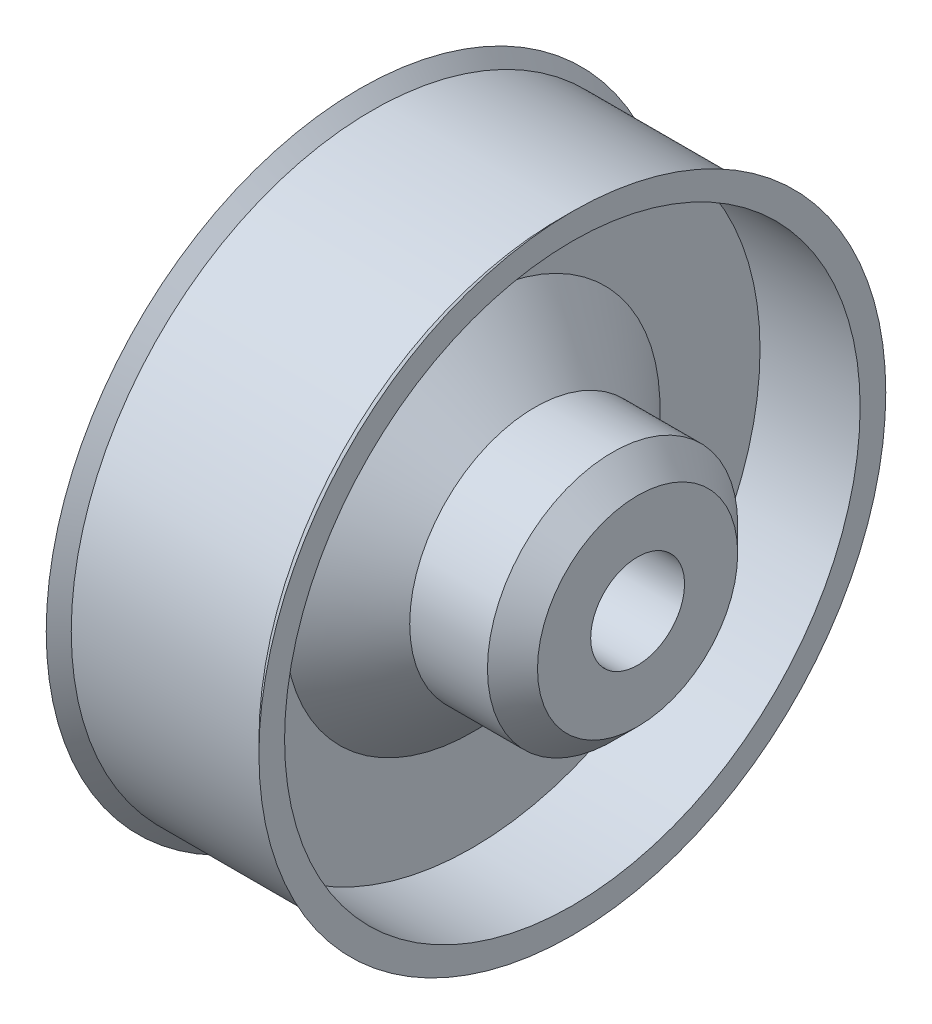
from build123d import *


with BuildPart() as part:
    # Sketch1 → Revolve1 (revolve)
    with BuildSketch(Plane.XY, mode=Mode.PRIVATE) as revolve1_sk:
        Polygon((-4.442951931, 5.01), (-4.442951931, 4.6), (-3.392951931, 4.6), (-3.392951931, 1.248035053), (-4.442951931, 0.813110813), (-4.55, 0), (-2.75, 0), (-2.75, 0.75), (0, 0.75), (0, 1.6), (-0.4, 2), (-1.642951931, 2), (-2.642951931, 3), (-2.642951931, 4.6), (-1.042951931, 4.6), (-1.042951931, 5.01), (-1.242951931, 4.81), (-4.242951931, 4.81), align=None)
    revolve(revolve1_sk.sketch.rotate(Axis((-2.75, 0, 0), (1, 0, 0)), 90), axis=Axis((-2.75, 0, 0), (1, 0, 0)))


solid = part.part
